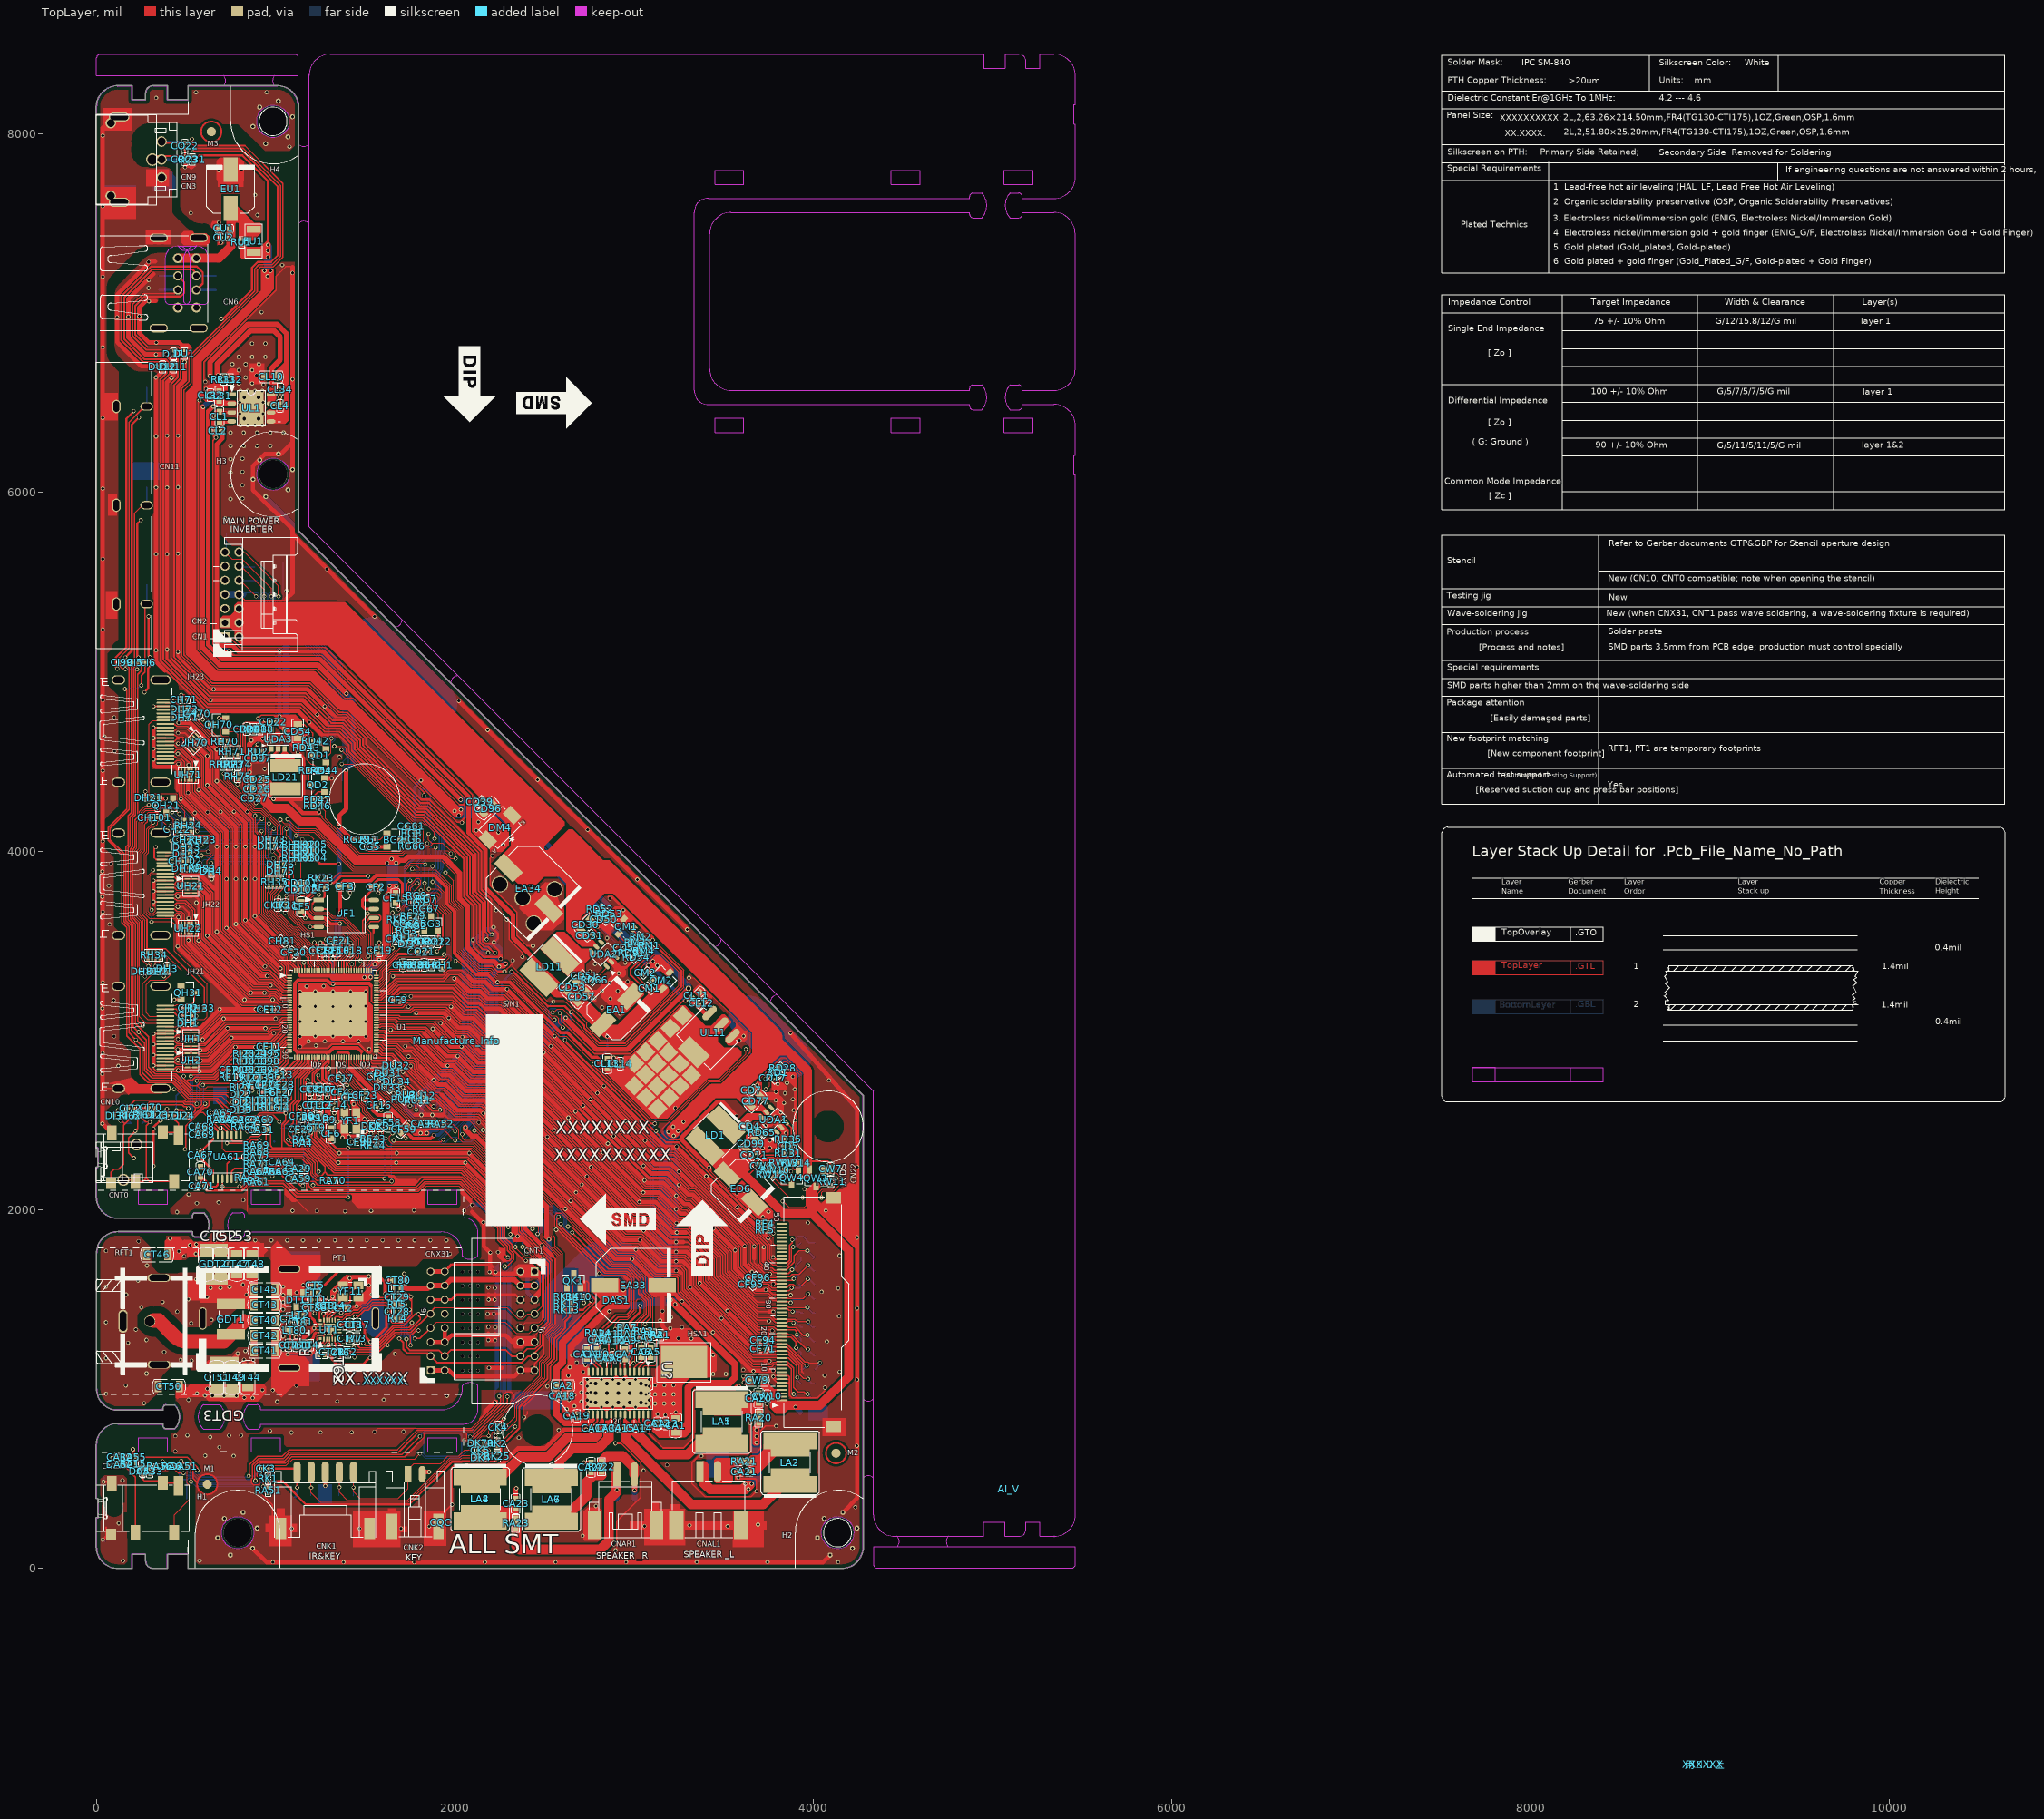
[diagram p0: TopLayer view]
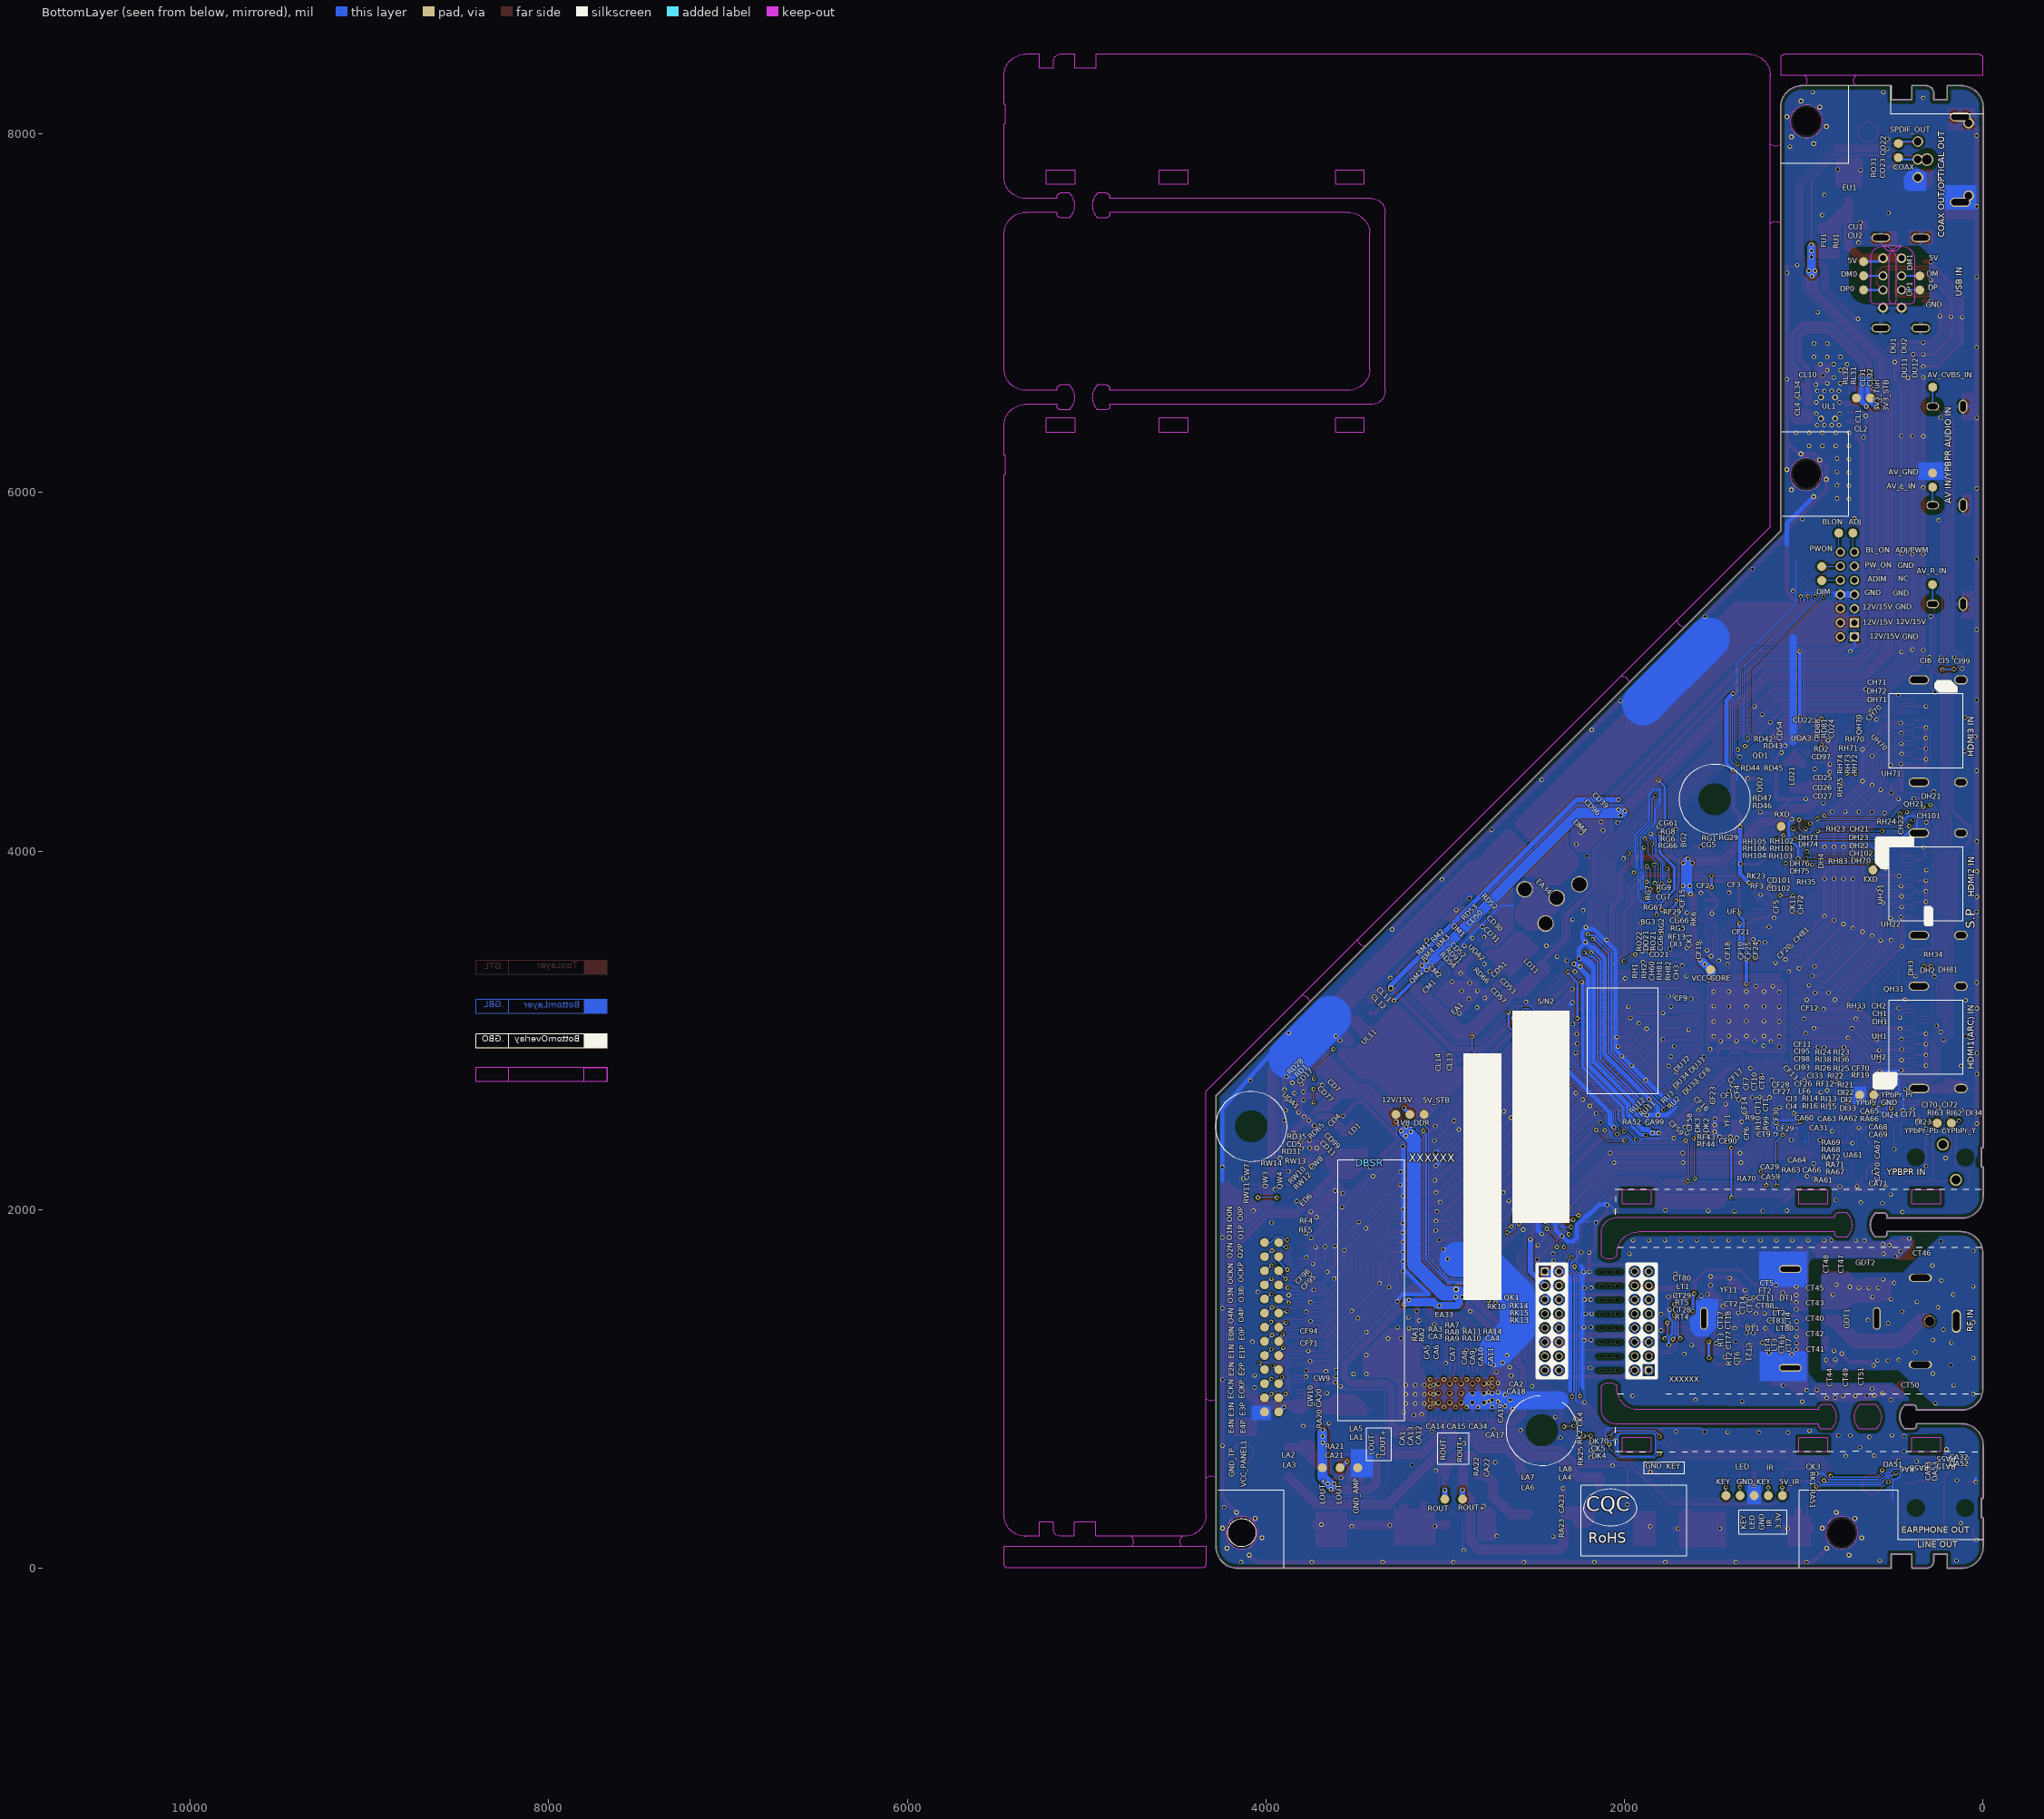
[diagram p1: BottomLayer view, seen from below]
# Altium PCB MISC105950.PcbDoc (part 1 of 15)
Units mil, origin at the board's own origin, x right, y up, seen from the top; angles counter-clockwise.
Board outline 4280.62 x 8272.76 mil, 2 copper layers (TopLayer, BottomLayer), stack 61.855 mil thick; 541 components, 268 nets, 2324 pads, 1157 vias.

## Layer stack, top to bottom
TopLayer: signal copper 1.4
Dielectric: core 59.055, FR-4, Dk 4.8
BottomLayer: signal copper 1.4

## Board outline
118.11,-2.52 cw(c118.11,118.11) -2.51,118.11 -2.51,279.53 cw(c0,279.53) 0,282.04 5.36,282.04 5.36,387.25 0,387.25 cw(c0,389.76) -2.51,389.76 -2.51,685.62 cw(c118.11,685.62) 118.11,806.24 368.5,806.24 cw(c368.5,803.73) 370.84,804.64 cw(c368.7,803.32) 371.22,803.32 371.22,793.82 ccw(c368.7,793.82) 371.22,793.84 371.22,793.82 ccw(c388.39,793.82) 388.39,776.65 434.98,776.65 ccw(c367.13,843.03) 462.05,843.03 ccw(c367.13,843.03) 434.98,909.42 388.39,909.42 ccw(c388.39,911.93) 388.41,909.42 388.39,909.42 ccw(c388.39,892.25) 371.22,892.25 cw(c368.7,892.25) 371.22,892.21 371.22,882.47 cw(c368.7,882.47) 368.6,879.95 cw(c368.5,882.47) 368.5,879.95 119.32,879.95 cw(c119.32,882.47) 119.28,879.95 ccw(c119.32,1000.58) 119.32,879.95 119.28,879.95 cw(c119.32,1000.58) -1.31,1000.54 cw(c119.32,1000.58) -1.31,1000.58 -1.31,1756.48 cw(c119.32,1756.48) 119.32,1877.11 532,1877.11 cw(c532,1874.59) 532.35,1877.08 cw(c532.7,1874.59) 535.22,1874.59 535.22,1864.75 ccw(c532.7,1864.75) 535.22,1864.78 535.22,1864.75 ccw(c552.39,1864.75) 552.39,1847.58 598.98,1847.58 ccw(c531.13,1913.96) 626.05,1913.96 ccw(c531.13,1913.96) 598.98,1980.35 552.39,1980.35 cw(c552.39,1982.86) 552.37,1980.35 cw(c552.39,1963.18) 552.39,1980.35 552.37,1980.35 ccw(c552.39,1963.18) 535.22,1963.18 cw(c532.7,1963.18) 535.22,1963.15 535.22,1953.33 cw(c532.7,1953.33) 532.35,1950.84 cw(c532,1953.33) 532,1950.82 118.11,1950.82 cw(c118.11,2071.44) -2.51,2071.44 -2.51,2236.22 cw(c0,2236.22) 0,2238.74 5.36,2238.74 5.36,2343.48 0,2343.48 cw(c0,2346) -2.5,2346.23 cw(c0,2346.46) -2.51,2346.46 -2.51,8153 cw(c0,8153) -2.45,8153.57 cw(c118.11,8149.62) 118.11,8270.24 cw(c118.11,8267.73) 118.13,8270.24 196.85,8270.24 cw(c196.85,8267.73) 199.37,8267.73 199.37,8191.5 273.08,8191.5 273.08,8228.36 cw(c314.96,8228.36) 314.96,8270.24 393.7,8270.24 cw(c393.7,8267.73) 396.22,8267.73 396.22,8191.5 509.3,8191.5 509.3,8267.68 cw(c511.81,8267.72) 509.3,8267.89 cw(c511.81,8267.73) 511.96,8270.24 1008.03,8270.24 1007.87,8270.24 ccw(c1007.87,8267.72) 1007.84,8270.24 1007.87,8270.24 cw(c1007.87,8149.61) 1128.5,8149.61 cw(c1125.99,8149.61) 1128.5,8149.59 1128.5,5786.06 4277.37,2637.19 cw(c4275.59,2635.41) 4278.11,2635.41 4278.11,118.11 ccw(c4275.59,118.11) 4278.11,118.13 4278.11,118.11 cw(c4157.48,118.11) 4157.48,-2.52 cw(c4157.48,0) 4157.46,-2.52 511.81,-2.52 cw(c511.81,0) 509.3,0 509.3,76.23 396.22,76.23 396.22,0 cw(c393.7,0) 393.7,-2.52 314.96,-2.52 cw(c314.96,39.37) 273.08,39.37 273.08,76.23 199.37,76.23 199.37,0 cw(c196.85,0) 196.85,-2.52

## Design rules (kind name [scope] priority, off if disabled: settings)
Clearance ■VIA2VIA_0.41mm_2 [((IsVia OR InPadClass('VIA5')) And Not ((IsVia OR InPadClass('VIA5')) And (AsMM(HoleDiameter) = 0.1))) And Not (WithInRoom('BGA0p65-1') OR WithInRoom('BGA0p65-2')) vs ((IsVia OR InPadClass('VIA5')) And Not ((IsVia OR InPadClass('VIA5')) And (AsMM(HoleDiameter) = 0.1))) And Not (WithInRoom('BGA0p65-1') OR WithInRoom('BGA0p65-2'))] p1: gap=16.14
Clearance ■VIA2VIA_10.2mil [(IsVia OR InPadClass('VIA5')) And Not ((IsVia OR InPadClass('VIA5')) And (AsMM(HoleDiameter) = 0.1)) vs (IsVia OR InPadClass('VIA5')) And Not ((IsVia OR InPadClass('VIA5')) And (AsMM(HoleDiameter) = 0.1))] p2: gap=10.2
Clearance ■KEEPOUT_18mil [(IsTrack Or IsArc) And (AsMM(Width) < 1) And IsKeepOut vs Not IsPad] p3: gap=18
Clearance ■DFM_NPTH_10mil [(IsPadHoleValid And (PadIsPlated=false) Or IsPad And ((AsMM(PadXSize_AllLayers) < 1) or (AsMM(PadYSize_AllLayers) < 1 )) And IsKeepout) OR HasFootprintPad('ASSE*','0') vs Not IsPad] p4: gap=10
Clearance ■DFM_20mil [(IsTrack or IsArc or IsPad) And IsKeepOut vs IsTrack or IsArc or InPoly] p5: gap=20
Clearance ■C_RJ45_2mm [InNetClass('RJ45') vs Not InNetClass('RJ45') AND InNet('*')] p6: gap=78.74
Clearance ■PWR_A12_8mil [((InNetClass('PWR_A12_8mil') or InNet('*12V*') or InNet('*24V*') or InNet('*PVCC*') or InNet('*19V*') or InNet('*AMP*POWER*') or InNet('*AMP*VCC*') or InNet('*LNB*')) And Not InNetClass('A12_8mil_EXC')) and Not IsPad vs Not InPoly] p7: gap=8
Clearance ■SIP2GND_8mil [HasFootprint('SIP*') vs InPoly] p8: gap=8
Clearance ■C_BGA_0P65 [HasFootprint('BGA*0.65*') vs InPoly] p9: gap=5
Clearance ■C_BGA_0P8 [HasFootprint('BGA*0.8*') vs InPoly] p10: gap=5.5
Clearance ■Poly_4mil [InPolygonClass('Poly_4mil') vs Not InPoly] p11: gap=4
Clearance ■Poly_5mil [InPolygonClass('Poly_5mil') vs Not InPoly] p12: gap=5
Clearance ■Poly_6.2mil [InPolygonClass('Poly_6.2mil') vs Not InPoly] p13: gap=6.2
Clearance ■Poly_8mil [InPolygonClass('Poly_8mil') vs Not InPoly] p14: gap=8
Clearance ■C_RFGND_1.8mm [InNet('RFGND') vs Not (InNet('RF*IN*') OR((IsTrack Or IsArc) And (AsMils(Width) < 6) And IsKeepOut) OR InNet('NetCT28*'))] p15: gap=70.87
Clearance ■ESD_10mil [HasFootprint('*IEC*') Or HasFootprint('*-F1*') Or HasFootprint('ANT-RF*')] p16: gap=10
Clearance ■ESD_20mil [HasFootprint('*SHIELD*')] p17: gap=20
Clearance ■GND_12mil [InNet('GND') vs InPoly] p18: gap=12
Clearance ■ESD_30mil [(HasFootprint('SCART*') OR HasFootprint('AV*') OR HasFootprint('DB15*') OR HasFootprint('PHONE*')) vs OnBottomLayer] p19: gap=30
Clearance ■ESD_NT_30mil [HasFootprint('SCART*') Or HasFootprint('PHONE-HD-12') Or HasFootprint('PHONE-HD-17') Or HasFootprint('PHONE-HD-10') Or HasFootprint('PHONE-HD-26') vs InNet('GND') And OnTopLayer] p20: gap=30
Clearance ■DFM_TH_5mil [HasFootprint('GND') or HasFootprint('TP*') or HasFootprint('MARK*') or HasFootprint('SPARK_GAP') or HasFootprint('USB-HD-3-2') or HasFootprint('PHONE-HS-20') and Not IsRegion vs OnBottomlayer And IsPad OR IsPadHoleValid] p21: gap=5
Clearance ■DFM_HS60_5mil [InPadClass('HS60') vs InPadClass('HS60') OR IsPadHoleValid and not InPadClass('VIA5')] p22: gap=5
Clearance ■DFM_BCR_4mm [IsPadHoleValid vs IsBoardCutoutRegion] p23: gap=157.48
Clearance ■DFM_TH_4mm [OnBottomlayer And IsSMTPin vs IsPadHoleValid and not InPadClass('VIA5')] p24: gap=157.48
Clearance ■DFM_HS60_4mm [InPadClass('HS60') vs IsPad and OnBottomlayer] p25: gap=157.48
Clearance ■V2V_BGA0p65_9p8mil [((IsVia OR InPadClass('VIA5')) And Not ((IsVia OR InPadClass('VIA5')) And (AsMM(HoleDiameter) = 0.1))) And (WithInRoom('BGA0p65-1') OR WithInRoom('BGA0p65-2')) vs ((IsVia OR InPadClass('VIA5')) And Not ((IsVia OR InPadClass('VIA5')) And (AsMM(HoleDiameter) = 0.1))) And (WithInRoom('BGA0p65-1') OR WithInRoom('BGA0p65-2'))] p26: gap=9.8
Clearance ■V2P_BGA0p65_4p7mil [HasFootprint('BGA*') and IsPad And (WithInRoom('BGA0p65-1') OR WithInRoom('BGA0p65-2')) vs (IsVia OR InPadClass('VIA5')) And Not (IsVia And (AsMM(HoleDiameter) = 0.1))] p27: gap=4.7
Clearance ■VIA2PAD_BGA_5mil [(HasFootprint('BGA*') and IsPad) And Not (WithInRoom('BGA0p65-1') OR WithInRoom('BGA0p65-2')) vs (IsVia OR InPadClass('VIA5')) And Not ((IsVia OR InPadClass('VIA5')) And (AsMM(HoleDiameter) = 0.1))] p28: gap=5
Clearance ■VIA2PAD_6mil [(IsVia OR InPadClass('VIA5')) And Not ((IsVia OR InPadClass('VIA5')) And (AsMM(HoleDiameter) = 0.1)) vs IsPad And Not HasFootprintPad('*','EPAD') and Not HasFootprintPad('*','257') and Not HasFootprintPad('TP','*') and Not HasFootprintPad('GND','JP*') and Not HasFootprintPad('LQFP216/0.4-2','217') and Not HasFootprintPad('QFP16*','17') and Not HasFootprintPad('QFN16*','17') and Not HasFootprintPad('QFN20*','21') and Not HasFootprintPad('QFN24*','25') and Not HasFootprintPad( 'QFN24*','29') and Not HasFootprintPad('QFN28*','29') and Not HasFootprintPad('QFN32*','33') and Not HasFootprintPad('QFN36*','37') and Not HasFootprintPad('QFN36*','0') and Not HasFootprintPad('QFN32*','0') and Not HasFootprintPad('QFN40*','41') and Not HasFootprintPad('QFN48*','49') and Not HasFootprintPad('LQFP48/0.5-2','49') and Not HasFootprintPad('*SSOP32*','33') and Not HasFootprintPad('SOP8*','9') and Not HasFootprintPad('WSON8/1.27*','9') and Not HasFootprintPad('DFN10/0.5-1*','11') and Not HasFootprintPad('SON16/0.4','9') and Not HasFootprintPad('MSOP10/0.5-1','11') and Not HasFootprintPad('QFN56/0.5','57') and Not HasFootprintPad('LGA31/0.5','3*') and Not InPadClass('VIA_HS60') and Not HasFootprintPad('TSSOP16/0.65-3','17') and Not HasFootprintPad('QFP128/0.5-2','129') and Not HasFootprintPad('QFP128/0.4-5','129') and Not HasFootprintPad('PQFP48*','49') and Not HasFootprintPad('QFP156/0.4-1','157') and Not HasFootprintPad('D2PAK3-TO-252','2') and Not HasFootprintPad('D2PAK3','2')] p29: gap=6
Clearance ■PAD2VIA5_6mil [(IsPad And Not (WithInRoom('BGA0p65-1') OR WithInRoom('BGA0p65-2'))) And ((AsMM(PadXSize_AllLayers) < 2.5) or ((AsMM(PadYSize_AllLayers) < 2.5))) And Not InPadclass('HS60') vs InPadClass('VIA5')] p30: gap=6
Clearance "■12mil for Polygon" [InPoly] p31: gap=12
Clearance 8mil [All] p32 off: gap=8
Clearance 7mil [All] p33 off: gap=7
Clearance 6.2mil [All] p34 off: gap=6.2
Clearance 6mil [All] p35 off: gap=6
Clearance 5.8mil [All] p36 off: gap=5.8
Clearance 5mil [Not ((IsTrack Or IsArc) And (Layer = 'KeepOutLayer')) vs Not (IsPad or ((IsTrack Or IsArc) And (Layer = 'KeepOutLayer')))] p37: gap=5
Clearance 4.5mil [Not ((IsTrack Or IsArc) And (Layer = 'KeepOutLayer')) vs Not (IsPad or ((IsTrack Or IsArc) And (Layer = 'KeepOutLayer')))] p38 off: gap=4.5
Clearance "4mil for Minimum" [Not ((IsTrack Or IsArc) And (Layer = 'KeepOutLayer')) vs Not (IsPad or ((IsTrack Or IsArc) And (Layer = 'KeepOutLayer')))] p39: gap=4
ComponentClearance ■DFMC_1mm [Not (InComponentClass('Co-Layout') Or HasFootprint('GND')) And (HasFootprint('T/E*') Or HasFootprint('T/PQ*') Or HasFootprint('USB*') Or HasFootprint('HDMI*') Or HasFootprint('USB*') Or HasFootprint('DC-*') Or HasFootprint('AV*') Or HasFootprint('ANT*') Or HasFootprint('PHONE*') Or HasFootprint('CICARD*') Or HasFootprint('CARD*') Or HasFootprint('DVI*') Or HasFootprint('DB*') Or HasFootprint('DP*') Or HasFootprint('DISPLAYPORT*') Or HasFootprint('OPTICAL*') Or HasFootprint('SCART*') Or HasFootprint('RJ45*') Or HasFootprint('USB*') Or HasFootprint('T-*') Or HasFootprint('T/*') Or HasFootprint('200-*') Or HasFootprint('ZhiJia*') Or HasFootprint('Dianpian*') Or HasFootprint('TanPian*') Or HasFootprint('P(*')) vs Not (InComponentClass('Co-Layout') Or HasFootprint('GND'))] p1 off: gap=39.37 collisioncheckmode=3 verticalgap=39.37 showdistances=FALSE
ComponentClearance ■DFMC_0.5mm [Not (InComponentClass('Co-Layout') Or HasFootprint('SO-23') Or HasFootprint('DIODE-s0402') Or HasFootprint('GND')) And (HasFootprint('M-*') Or HasFootprint('BGA*') Or HasFootprint('QFP*') Or HasFootprint('QFN*') Or HasFootprint('*DFN*') Or HasFootprint('*SOP*') Or HasFootprint('LGA*') Or HasFootprint('SOIC*') Or HasFootprint('EC*') Or HasFootprint('AC-*') Or HasFootprint('DIODE*') Or HasFootprint('XTAL*') Or HasFootprint('SO-*') Or HasFootprint('L/LC*') Or HasFootprint('L(*') Or HasFootprint('WIFI*') Or HasFootprint('SATA*') Or HasFootprint('POGO*') Or HasFootprint('SOT-223') Or HasFootprint('TO-252') Or HasFootprint('TO-263') Or HasFootprint('KEY*') Or HasFootprint('SW*') Or HasFootprint('DIP*') Or HasFootprint('SIP*') Or HasFootprint('DIP*') Or HasFootprint('CON*') Or HasFootprint('FFC*') Or HasFootprint('FPC*') Or HasFootprint('GDT*') Or HasFootprint('R2512*') Or HasFootprint('R2725*') Or HasFootprint('L2012*') Or HasFootprint('L2520*')) vs Not (InComponentClass('Co-Layout') Or HasFootprint('SO-23') Or HasFootprint('DIODE-s0402') Or HasFootprint('GND'))] p2 off: gap=19.68 collisioncheckmode=3 verticalgap=19.68 showdistances=FALSE
ComponentClearance ■DFMC_0.4mm [Not (InComponentClass('Co-Layout') Or HasFootprint('GND')) And (HasFootprint('C0201*') Or HasFootprint('C0402*') Or HasFootprint('C0603*') Or HasFootprint('C0805*') Or HasFootprint('C1206*') Or HasFootprint('C1210*') Or HasFootprint('R0201*') Or HasFootprint('R0402*') Or HasFootprint('R0603*') Or HasFootprint('R0805*') Or HasFootprint('R*0402*') Or HasFootprint('L0201*') Or HasFootprint('L0402*') Or HasFootprint('L0603*') Or HasFootprint('L0805*') Or HasFootprint('L1206*') Or HasFootprint('DIODE-s0402')) vs Not (InComponentClass('Co-Layout') Or HasFootprint('GND')) And (HasFootprint('C0201*') Or HasFootprint('C0402*') Or HasFootprint('C0603*') Or HasFootprint('C0805*') Or HasFootprint('C1206*') Or HasFootprint('C1210*') Or HasFootprint('R0201*') Or HasFootprint('R0402*') Or HasFootprint('R0603*') Or HasFootprint('R0805*') Or HasFootprint('R*0402*') Or HasFootprint('L0201*') Or HasFootprint('L0402*') Or HasFootprint('L0603*') Or HasFootprint('L0805*') Or HasFootprint('L1206*') Or HasFootprint('DIODE-s0402'))] p3 off: gap=15.75 collisioncheckmode=3 verticalgap=15.75 showdistances=FALSE
ComponentClearance ■DFMC_0.36mm [Not (InComponentClass('Co-Layout') Or HasFootprint('GND')) And HasFootprint('R1206*') vs Not (InComponentClass('Co-Layout') Or HasFootprint('GND')) And HasFootprint('R1206*')] p4 off: gap=14.17 collisioncheckmode=3 verticalgap=14.17 showdistances=FALSE
ComponentClearance ■DFMC_0.25mm [Not (InComponentClass('Co-Layout') Or HasFootprint('GND')) vs Not (InComponentClass('Co-Layout') Or HasFootprint('GND'))] p5 off: gap=9.84 collisioncheckmode=3 verticalgap=9.84 showdistances=FALSE
DiffPairsRouting ■DiffPair_USB_DiffPairsRouting [InDifferentialPairClass('USB')] p1: maxlimit=5 minlimit=4 mostfreqgap=5 maxuncoupledlength=200
DiffPairsRouting ■DiffPair_LVDS_DiffPairsRouting [InDifferentialPairClass('LVDS')] p2: maxlimit=5 minlimit=4 mostfreqgap=5 maxuncoupledlength=500
DiffPairsRouting ■DiffPair_HDMI_DiffPairsRouting [InDifferentialPairClass('HDMI')] p3: maxlimit=5 minlimit=4 mostfreqgap=5 maxuncoupledlength=200
DiffPairsRouting [All] p4: maxlimit=10 minlimit=10 mostfreqgap=10 maxuncoupledlength=500
FabricationTestPointUsage TestPointUsage [All] p1: valid=0 allowmultiple=FALSE
FabricationTestpoint Testpoint [All] p1: side=3 testpointundercomponent=TRUE minsize=40 maxsize=100 preferedsize=60 minholesize=20 maxholesize=40 preferedholesize=32 testpointgrid=1 allowsidetop=TRUE allowsidebottom=TRUE usegrid=TRUE gridtolerance=0.01
HoleSize HoleSize_VIA [ISVIA] p1 off: absolutevalues=TRUE maxlimit=23.62 minlimit=7.87 maxpercent=80.000 minpercent=20.000
HoleToHoleClearance Hole2Hole [All] p1 off: gap=18 allowstackedmicrovias=FALSE
MatchedLengths DiffPair_USB_MatchedLengths [InDifferentialPairClass('USB')] p1: tolerance=100 checknetsindiffpair=TRUE checkdiffpairvsdiffpair=TRUE checkothers=TRUE
MatchedLengths DiffPair_LVDS_MatchedLengths [InDifferentialPairClass('LVDS')] p2: tolerance=100 checknetsindiffpair=TRUE checkdiffpairvsdiffpair=TRUE checkothers=TRUE
MatchedLengths DiffPair_HDMI_MatchedLengths [InDifferentialPairClass('HDMI')] p3: tolerance=100 checknetsindiffpair=TRUE checkdiffpairvsdiffpair=TRUE checkothers=TRUE
MinimumAnnularRing [All] p1: minimumring=3.94
MinimumSolderMaskSliver ■MiniSolderMaskSliver [All] p1 off: minsoldermaskwidth=3.87
NetAntennae [Not (HasFootprint('ANT-7') or HasFootprint('ANT-BLUECORE'))] p1: netantennaetolerance=40
PermittedLayers [All] p1: toplayerpermitted=TRUE bottomlayerpermitted=TRUE
PlaneClearance ■Plane_ESD_30mil [(HasFootprint('SCART*') OR HasFootprint('AV*') OR HasFootprint('DB15*') OR HasFootprint('PHONE*'))] p1: clearance=30
PlaneClearance ■Plane_All_9mil [All] p2: clearance=9
PlaneConnect ■PlaneOverAll [IsVia or InPadClass('VIA5') Or HasFootprint('ASSE*') OR InPadclass('HS60')] p1: planeconnectstyle=Direct reliefexpansion=20 reliefentries=4 reliefconductorwidth=10 reliefairgap=10
PlaneConnect ■PlaneConnect [All] p2: planeconnectstyle=Relief reliefexpansion=12 reliefentries=4 reliefconductorwidth=30 reliefairgap=12
PolygonConnect ■PourOverAll [IsVia Or InPadclass('HS60') Or InPadClass('VIA5') Or HasFootprint('ASSE*') Or HasFootprint('DIODE-S0402') Or HasFootprint('RCL0524P') Or HasFootprint('SOT-89') OR HasFootprint('SOT-223') OR HasFootprint('TO-252') OR HasFootprint('TO-263') OR HasFootprint('DIODE') OR HasFootprint('SW-HS-2') OR HasFootprint('HDMI*') OR HasFootprint('SO-8B') OR HasFootprint('GND') OR HasFootprint('PHONE*') OR HasFootprint('DIP18/2.54-2') OR HasFootprint('DIP18/2.54-1') OR HasFootprint('UFL-R-SMT-1') OR HasFootprint('WIFI') OR HasFootprint('UM02BS') OR HasFootprint('*SCART*') OR HasFootprint('TSOT23-8/0.65') OR HasFootprint('*SOT-23-*') OR HasFootprint('SOP23-5-1') OR HasFootprint('SOP6/0.95') OR HasFootprint('M-WIFI-2-M603USA1') OR HasFootprint('M-MT7632U') OR HasFootprint('SOP8/1.27') OR HasFootprint('SOP8/1.27-3') OR HasFootprint('TSOT23-6') vs IsPolygon] p1: connectstyle=Direct reliefconductorwidth=10 reliefentries=4 polygonreliefangle="90 Angle"
PolygonConnect ■BGA_0P65 [HasFootprint('BGA*0.65*') vs IsPoly] p2: connectstyle=Relief reliefconductorwidth=8 reliefentries=4 polygonreliefangle="45 Angle"
PolygonConnect ■BGA_0P8 [HasFootprint('BGA*0.8*') vs IsPoly] p3: connectstyle=Relief reliefconductorwidth=9 reliefentries=4 polygonreliefangle="45 Angle"
PolygonConnect ■Polygon_RFGND [InNet('RFGND')] p4: connectstyle=Direct reliefconductorwidth=10 reliefentries=4 polygonreliefangle="90 Angle"
PolygonConnect ■ESD_SCART [HasFootprint('SCART*') vs IsPolygon And onBottomlayer] p5: connectstyle=Direct reliefconductorwidth=30 reliefentries=4 polygonreliefangle="90 Angle"
PolygonConnect ■C2Polygon_35mil [HasFootprint('EC*') vs IsPolygon] p6: connectstyle=Relief reliefconductorwidth=35 reliefentries=4 polygonreliefangle="90 Angle"
PolygonConnect ■C2Polygon_30mil [(HasFootprint('*0805*') OR HasFootprint('*1206*')) vs IsPolygon] p7: connectstyle=Relief reliefconductorwidth=30 reliefentries=4 polygonreliefangle="90 Angle"
PolygonConnect ■C2Polygon_25mil [HasFootprint('*0603*') Or IsThruPin vs IsPolygon] p8: connectstyle=Relief reliefconductorwidth=25 reliefentries=4 polygonreliefangle="90 Angle"
PolygonConnect ■C2Polygon_12mil [IsSMTPin vs IsPolygon] p9: connectstyle=Relief reliefconductorwidth=12 reliefentries=4 polygonreliefangle="90 Angle"
RoutingVias 0.6_0.4 [All] p1: holewidth=15.75 width=23.62 viastyle="Through Hole" minholewidth=15.75 minwidth=23.62 maxholewidth=15.75 maxwidth=23.62
RoutingVias 0.8_0.5 [All] p2 off: holewidth=19.68 width=31.5 viastyle="Through Hole" minholewidth=19.68 minwidth=31.5 maxholewidth=19.68 maxwidth=31.5
RoutingVias 0.5_0.3 [All] p3 off: holewidth=11.81 width=19.68 viastyle="Through Hole" minholewidth=11.81 minwidth=19.68 maxholewidth=11.81 maxwidth=19.68
RoutingVias 0.45_0.25 [All] p4 off: holewidth=9.84 width=17.72 viastyle="Through Hole" minholewidth=9.84 minwidth=17.72 maxholewidth=9.84 maxwidth=17.72
RoutingVias 0.4_0.2 [All] p5 off: holewidth=7.87 width=15.75 viastyle="Through Hole" minholewidth=7.87 minwidth=15.75 maxholewidth=7.87 maxwidth=15.75
RoutingVias 0.25_0.1 [All] p6 off: holewidth=3.94 width=9.84 viastyle="Through Hole" minholewidth=3.94 minwidth=9.84 maxholewidth=3.94 maxwidth=9.84
SMDNeckDown ■SMDNeckDown_Chip [HasFootprint('FFC*') or HasFootprint('QFP*') or HasFootprint('QFN*') or HasFootprint('HDMI*') or HasFootprint('BGA*')] p1: percent=100.000
SMDToCorner [All] p1 off: distance=40000
ShortCircuit ■ShortCircuit_ViaOnEpad [HasFootprintPad( '*','EPAD') vs IsVia AND InNet('*')] p1: allowed=TRUE
ShortCircuit ■ShortCircuit_JP [HasFootprintPad( 'GND','JP_1K') vs HasFootprintPad( 'GND','JP_2K')] p2: allowed=TRUE
ShortCircuit ■ShortCircuit_R0402 [HasFootprintPad('R0402SC','1') OR HasFootprintPad('R0402SC','2') vs HasFootprintPad('R0402SC','3')] p3: allowed=TRUE
ShortCircuit ■ShortCircuit_R0603 [HasFootprintPad('R0603SC','1') OR HasFootprintPad('R0603SC','2') vs HasFootprintPad('R0603SC','3')] p4: allowed=TRUE
ShortCircuit ■ShortCircuit_R0805 [HasFootprintPad('R0805SC','1') OR HasFootprintPad('R0805SC','2') vs HasFootprintPad('R0805SC','3')] p5: allowed=TRUE
ShortCircuit ■ShortCircuit_L0805 [HasFootprintPad('L0805SC','1') OR HasFootprintPad('L0805SC','2') vs HasFootprintPad('L0805SC','3')] p6: allowed=TRUE
ShortCircuit ■ShortCircuit_R1206 [HasFootprintPad('R1206SC','1') OR HasFootprintPad('R1206SC','2') vs HasFootprintPad('R1206SC','3')] p7: allowed=TRUE
ShortCircuit ■ShortCircuit [InNet('*')] p8: allowed=FALSE
SilkToSilkClearance ■Silk2Silk [All] p1: silktosilkclearance=5
SilkscreenOverComponentPads ■SilkOverPads [IsText] p1: minsilkscreentomaskgap=0.1
SolderMaskExpansion ■SolderMask_VIA [IsVia] p1: expansion=5.1
SolderMaskExpansion ■SolderMask_All [All] p2: expansion=2
UnRoutedNet ■UnRoutedNet [All] p1:
ViasUnderSMD [All] p1: allowed=FALSE
Width ■Width_2.5mm [InFromToClass('Width_2.5mm')] p1: maxlimit=98.43 minlimit=98.43 preferedwidth=98.43
Width ■Width_1.5mm [InFromToClass('Width_1.5mm')] p2: maxlimit=59.06 minlimit=59.06 preferedwidth=59.06
Width ■DiffPair_USB_Width [InDifferentialPairClass('USB')] p3: maxlimit=11 minlimit=4 preferedwidth=11
Width ■DiffPair_LVDS_Width [InDifferentialPairClass('LVDS')] p4: maxlimit=7 minlimit=4 preferedwidth=7
Width ■DiffPair_HDMI_Width [InDifferentialPairClass('HDMI')] p5: maxlimit=7 minlimit=4 preferedwidth=7
Width [All] p6: maxlimit=500 minlimit=3 preferedwidth=8
14 further rules are at their usual default settings.

## Classes and differential pairs
polygon class Poly_5mil: 5
pad class HS60: Free-HS60
pad class VIA5: Free-0 Free-VIA5
component class PCB_info: AI_V CQC DAS1 H1 H2 H3 H4 M1 M2 M3 M4 Manufacture_Info S/N1 S/N2
component class SCH_info: DBSR HS1 XXXXXX XXXXXXXX XXXXXXXXXX 用U1上
component class TV#02_POWER: 1V8_DDR 3V3_STB 3V3_Tun 5V_STB 12V/15V ADJ BG2 BG3 BLON CD4 CD5 CD7 CD11 CD17 CD22 CD24 CD25 CD26 CD27 CD30 CD31 CD39 CD50 CD51 CD52 CD53 CD54 CD57 CD77 CD96 CD97 CD99 CG5 CG6 CG7 CG61 CG66 CL1 CL2 CL4 CL10 CL11 CL12 CL13 CL14 CL31 CL32 CL34 CM1 CM2 CN1 CN2 DI3 DIM DM4 EA1 EA34 ED6 LD1 LD11 LD21 PWON QD1 QD2 QM1 QM2 RD1 RD2 RD28 RD31 RD35 RD42 RD43 RD44 RD45 RD46 RD47 RD52 RD53 RD54 RD65 RD66 RD81 RD88 RD91 RG1 RG2 RG3 RG6 RG7 RG8 RG9 RG29 RG66 RG67 RL31 RL32 RM1 RM2 RM3 RM4 UDA1 UDA2 UDA3 UL1 UL11 VCC_CORE
component class TV#03_V53: CF1 CF2 CF3 CF4 CF5 CF6 CF7 CF8 CF9 CF10 CF11 CF12 CF13 CF14 CF15 CF16 CF17 CF18 CF19 CF20 CF21 CF23 CF24 CF25 CF26 CF27 CF28 CF29 CF30 CF58 CF59 CF70 CF90 DK2 DK3 LF6 R9 RF3 RF12 RF13 RF19 RF29 RF43 RF44 U1 UF1 YF1
component class TV#04_IR&KEY: 5V_IR CK1 CK3 CK4 CK5 CK11 CNK1 CNK2 DK4 DK70 GND_KEY IR KEY LED QK1 RK1 RK2 RK6 RK10 RK13 RK14 RK15 RK23 RK25
component class TV#05_LVDS: CF71 CF94 CF95 CF96 CF97 CF98 CF99 CN22 CW7 CW8 CW9 CW10 E0N E0P E1N E1P E2N E2P E3N E3P E4N E4P ECKN ECKP GND_TP O0N O0P O1N O1P O2N O2P O3N O3P O4N O4P OCKN OCKP QW3 QW4 RF4 RF5 RW10 RW11 RW12 RW13 RW14 VCC_PANEL1
component class TV#06_INPUT: 5V AV_CVBS_IN AV_GND AV_L_IN AV_R_IN CI3 CI4 CI5 CI6 CI33 CI70 CI71 CI72 CI93 CI95 CI98 CI99 CN3 CN6 CN9 CN10 CN11 CNT0 CO21 CO22 CO23 COAX CU1 CU2 DI2 DI3 DI22 DI23 DI24 DI33 DI34 DM0 DM1 DO21 DP0 DP1 DU1 DU2 DU11 DU12 DU31 DU32 DU33 DU34 EU1 FU1 RI13 RI14 RI15 RI16 RI21 RI22 RI23 RI24 RI25 RI26 RI36 RI38 RI62 RI63 RO21 RO22 RO31 RU1 RU2 RU3 RU11 RU12 SPDIF_OUT YPbPr_GND YPbPr_Pb YPbPr_Pr YPbPr_Y
component class TV#07_HDMI: CD101 CD102 CH1 CH2 CH3 CH21 CH22 CH60 CH70 CH71 CH72 CH81 CH101 CH102 DH1 DH2 DH3 DH4 DH21 DH22 DH23 DH70 DH71 DH72 DH73 DH74 DH75 DH76 DH81 JH21 JH22 JH23 QH21 QH31 QH70 RH1 RH2 RH23 RH24 RH33 RH34 RH35 RH70 RH71 RH72 RH73 RH74 RH75 RH81 RH82 RH83 RH101 RH102 RH103 RH104 RH105 RH106 RXD TXD UH1 UH2 UH21 UH22 UH70 UH71
component class TV#08_AMP: CA1 CA2 CA3 CA4 CA5 CA6 CA7 CA8 CA9 CA10 CA11 CA12 CA13 CA14 CA15 CA17 CA18 CA19 CA20 CA21 CA22 CA23 CA34 CNAL1 CNAR1 EA33 GND_AMP HSA1 LA1 LA2 LA3 LA4 LA5 LA6 LA7 LA8 LOUT+ LOUT- RA1 RA2 RA3 RA4 RA5 RA7 RA8 RA9 RA10 RA11 RA14 RA20 RA21 RA22 RA23 ROUT+ ROUT- U?
component class TV#11_XX.XXXX: CNX31 CT1 CT2 CT3 CT4 CT5 CT6 CT7 CT8 CT9 CT10 CT11 CT12 CT14 CT17 CT18 CT21 CT28 CT29 CT40 CT41 CT42 CT43 CT44 CT45 CT46 CT47 CT48 CT49 CT50 CT51 CT52 CT53 CT61 CT62 CT77 CT80 CT81 CT88 DT1 FT2 GDT1 GDT2 GDT3 LT1 LT2 LT3 LT4 LT80 PT1 RFT1 RT1 RT2 RT3 RT4 RT5 UT1 XX.XXXX XXXXXX. YF11
component class TV#9_EARPHONE&LINEOUT: CA29 CA31 CA32 CA33 CA59 CA60 CA63 CA64 CA65 CA66 CA67 CA68 CA69 CA70 CA71 CA99 CN12 DA51 DA52 DA53 EPH_DET EPH_L EPH_R GND RA6 RA15 RA51 RA52 RA55 RA56 RA61 RA62 RA63 RA64 RA65 RA66 RA67 RA68 RA69 RA70 RA71 RA72 UA61
component class TV#10_TUNER_BOARD: CNT1 CT1 CT8 CT9 CT10 CT12 R10 R99

## Components (designator, comment, footprint, x,y, rotation, side; value= is the part's Value field where it differs from the comment)
1V8_DDR "TEST" TP 3195.74,2530.5 r270 bottom
3V3_STB "TEST" TP 626.63,6527.13 r270 bottom
3V3_Tun "TEST" TP 705.37,6527.13 r270 bottom
5V "DM0" TP 664.87,7288.12 r180 bottom
5V_IR "DM0" TP 1117.52,403.88 r90 bottom
5V_STB "TEST" TP 3117,2530.5 r180 bottom
12V/15V "TEST" TP 3274.48,2530.5 r0 bottom
ADJ "TEST" TP 724.76,5774.51 r90 bottom
AI_V "AI_GRIPPER_V" AI_GRIPPER_V 5092,440 r270 top
AV_CVBS_IN "TEST" TP 279.5,6588 r180 bottom
AV_GND "TEST" TP 280,6109.11 r180 bottom
AV_L_IN "TEST" TP 280,6030.37 r180 bottom
AV_R_IN "TEST" TP 280.5,5486.87 r180 bottom
BG2 "General-purpose transistor, Dynatron, NPN, 0.2A, 40V, 30-300, SOT-23, LMBT3904LT1G, LRC" SOT-23 1660.5,4061.5 r90 top